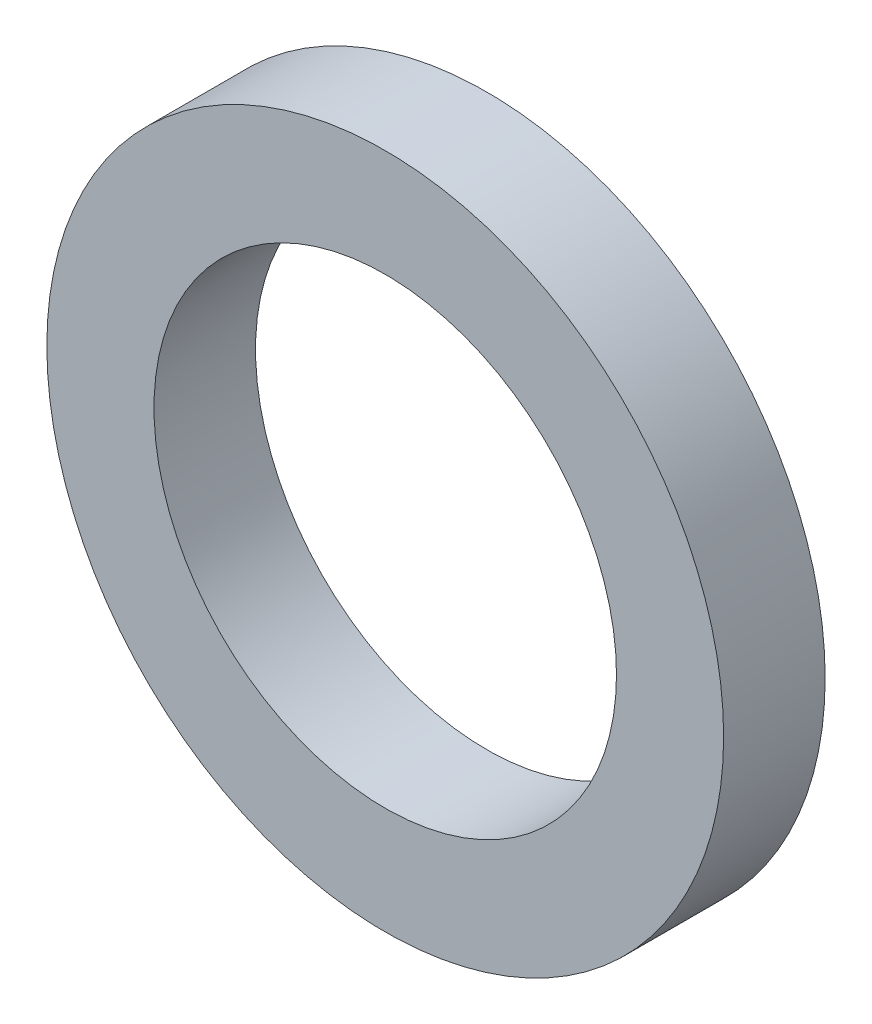
from build123d import *

# Parameters (mm, degrees)
SKETCH_1_R      = 15
SKETCH_1_R_2    = 10.25
EXTRUDE_1_DEPTH = 4.5


with BuildPart() as part:
    # 草图1 → 凸台-拉伸1 (new body)
    with BuildSketch(Plane.XY):
        Circle(SKETCH_1_R)
        Circle(SKETCH_1_R_2, mode=Mode.SUBTRACT)
    extrude(amount=EXTRUDE_1_DEPTH)


solid = part.part
